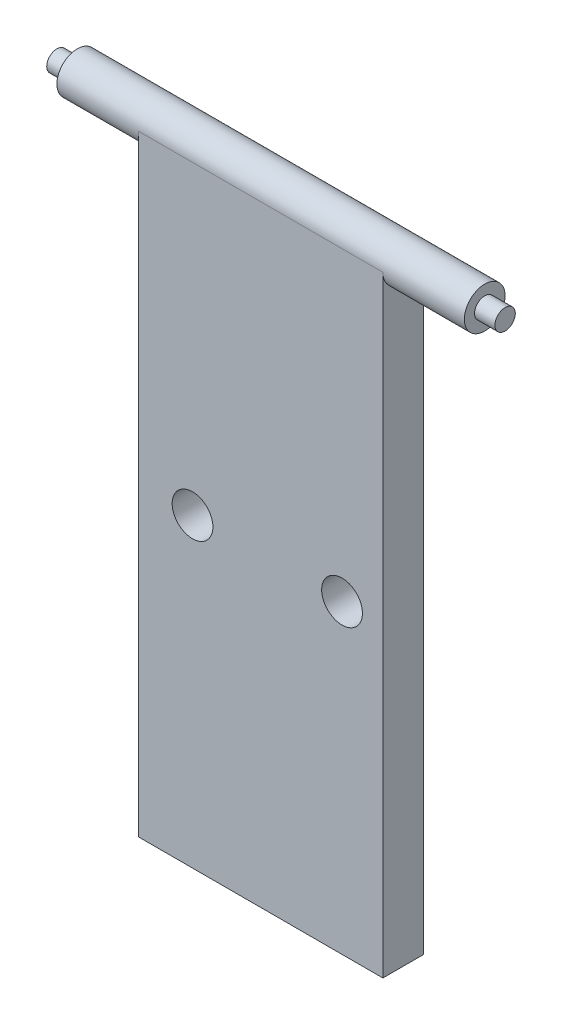
SolidWorks part; units mm, degrees
material "PVC Rigid"
ref_plane "Front Plane" through (0, 0, 0) normal (0, 0, 1) x (1, 0, 0)
ref_plane "Top Plane" through (0, 0, 0) normal (0, 1, 0) x (1, 0, 0)
ref_plane "Right Plane" through (0, 0, 0) normal (1, 0, 0) x (0, 0, -1)
sketch "Sketch1" plane through (0, 0, 0) normal (0, 0, 1) x (1, 0, 0)
  line L1 (30, -75) -> (-30, -75)
  line L2 (30, -75) -> (30, 75)
  line L3 (30, 75) -> (-30, 75)
  line L4 (-30, -75) -> (-30, 75)
  line L5 (30, -75) -> (-30, 75) construction
  line L6 (30, 75) -> (-30, -75) construction
  point P0 (0, 0)
  dimension "D1" = 150
  dimension "D2" = 60
extrude "Boss-Extrude1" add sketch "Sketch1" along normal blind 10
sketch "Sketch2" plane through (0, 0, 10) normal (0, 0, 1) x (1, 0, 0)
  circle A0 centre (-16.7175, 0) radius 5
  circle A1 centre (19.9764, 0) radius 5
  dimension "D1" = 10
  dimension "D2" = 10
extrude "Cut-Extrude1" cut sketch "Sketch2" against normal blind 10
sketch "Sketch3" plane through (30, 0, 0) normal (1, 0, 0) x (0, 0, -1)
  line L0 (-10, 75) -> (0, 75) construction
  circle A0 centre (-5, 75) radius 5
  dimension "D1" = 10
extrude "Boss-Extrude2" add sketch "Sketch3" along normal blind 20 and the other way blind 80.0001
sketch "Sketch4" plane through (-50.0001, 0, 0) normal (-1, 0, 0) x (0, 0, 1)
  circle A0 centre (5, 75) radius 2.5
  dimension "D1" = 5
extrude "Boss-Extrude3" add sketch "Sketch4" along normal blind 5 and the other way blind 105
